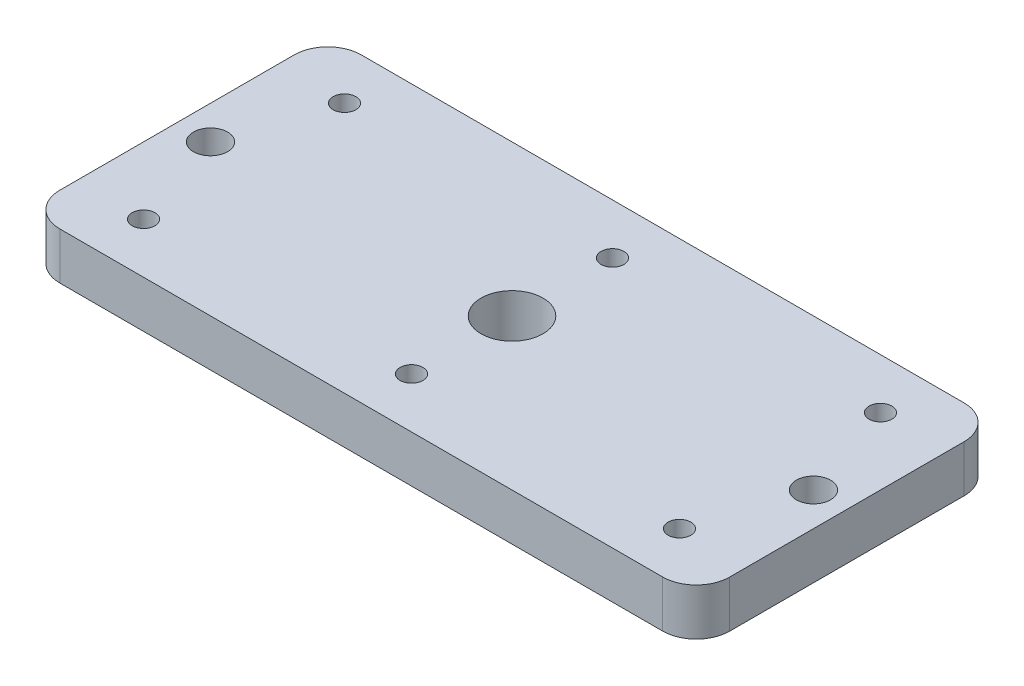
from build123d import *

# Parameters (mm, degrees)
SKETCH1_W              = 200
SKETCH1_H              = 90
BOSS_EXTRUDE1_DEPTH    = 14
M12_TAPPED_HOLE1_D     = 10.2
M12_TAPPED_HOLE1_DEPTH = 29.25
M12_TAPPED_HOLE1_TIP   = 3.064389157
FILLET1_R              = 10
M20X1_5_TAPPED_HOLE1_D = 18.5
M8_TAPPED_HOLE1_D      = 6.8


with BuildPart() as part:
    # Sketch1 → Boss-Extrude1 (new body)
    with BuildSketch(Plane(origin=(0, 0, 0), x_dir=(1, 0, 0), z_dir=(0, 1, 0))):
        with Locations((100, 45)):
            Rectangle(SKETCH1_W, SKETCH1_H)
    extrude(amount=BOSS_EXTRUDE1_DEPTH)

    # M12 Tapped Hole1
    with Locations(Plane(origin=(0, 14, 0), x_dir=(1, 0, 0), z_dir=(0, 1, 0))):
        with Locations((10, 45), (190, 45)):
            Hole(M12_TAPPED_HOLE1_D / 2, depth=M12_TAPPED_HOLE1_DEPTH)
            with Locations((0, 0, -(M12_TAPPED_HOLE1_DEPTH + M12_TAPPED_HOLE1_TIP / 2))):  # 118° drill point
                Cone(0, M12_TAPPED_HOLE1_D / 2, M12_TAPPED_HOLE1_TIP, mode=Mode.SUBTRACT)

    # Fillet1
    fillet1_edges = [part.edges().sort_by_distance(p)[0] for p in [
        (0, 7, -90),
        (200, 7, -90),
        (200, 7, 0),
        (0, 7, 0),
    ]]
    fillet(fillet1_edges, radius=FILLET1_R)

    # M20x1.5 Tapped Hole1 (through all)
    with Locations(Plane(origin=(0, 14, 0), x_dir=(1, 0, 0), z_dir=(0, 1, 0))):
        with Locations((100, 45)):
            Hole(M20X1_5_TAPPED_HOLE1_D / 2)

    # M8 Tapped Hole1 (through all)
    with Locations(Plane(origin=(0, 14, 0), x_dir=(1, 0, 0), z_dir=(0, 1, 0))):
        with Locations((20, 75), (100, 75), (180, 75), (180, 15), (100, 15), (20, 15)):
            Hole(M8_TAPPED_HOLE1_D / 2)


solid = part.part
